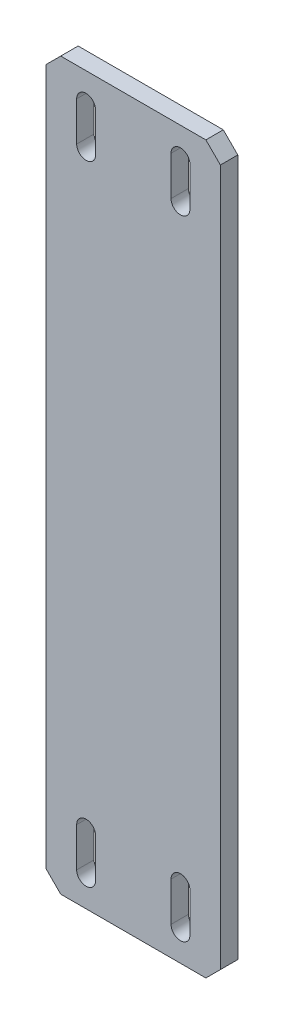
from build123d import *

# Parameters (mm, degrees)
SKETCH1_W           = 120
SKETCH1_H           = 500
BOSS_EXTRUDE1_DEPTH = 12
CUT_EXTRUDE1_DEPTH  = 12
CHAMFER1_SIZE       = 10


with BuildPart() as part:
    # Sketch1 → Boss-Extrude1 (new body)
    with BuildSketch(Plane.XY):
        Rectangle(SKETCH1_W, SKETCH1_H)
    extrude(amount=BOSS_EXTRUDE1_DEPTH)

    # Sketch2 → Cut-Extrude1 (cut)
    with BuildSketch(Plane.XY.offset(12)):
        with BuildLine():
            Line((-26, 230), (-26, 203))
            ThreePointArc((-26, 203), (-32.5, 196.5), (-39, 203))
            Line((-39, 203), (-39, 230))
            ThreePointArc((-39, 230), (-32.5, 236.5), (-26, 230))
        make_face()
        with BuildLine():
            Line((26, 230), (26, 203))
            ThreePointArc((26, 203), (32.5, 196.5), (39, 203))
            Line((39, 203), (39, 230))
            ThreePointArc((39, 230), (32.5, 236.5), (26, 230))
        make_face()
        with BuildLine():
            Line((26, -230), (26, -203))
            ThreePointArc((26, -203), (32.5, -196.5), (39, -203))
            Line((39, -203), (39, -230))
            ThreePointArc((39, -230), (32.5, -236.5), (26, -230))
        make_face()
        with BuildLine():
            Line((-26, -230), (-26, -203))
            ThreePointArc((-26, -203), (-32.5, -196.5), (-39, -203))
            Line((-39, -203), (-39, -230))
            ThreePointArc((-39, -230), (-32.5, -236.5), (-26, -230))
        make_face()
    extrude(amount=-CUT_EXTRUDE1_DEPTH, mode=Mode.SUBTRACT)

    # Chamfer1
    chamfer1_edges = [part.edges().sort_by_distance(p)[0] for p in [
        (60, -250, 6),
        (-60, -250, 6),
        (-60, 250, 6),
        (60, 250, 6),
    ]]
    chamfer(chamfer1_edges, length=CHAMFER1_SIZE)


solid = part.part
